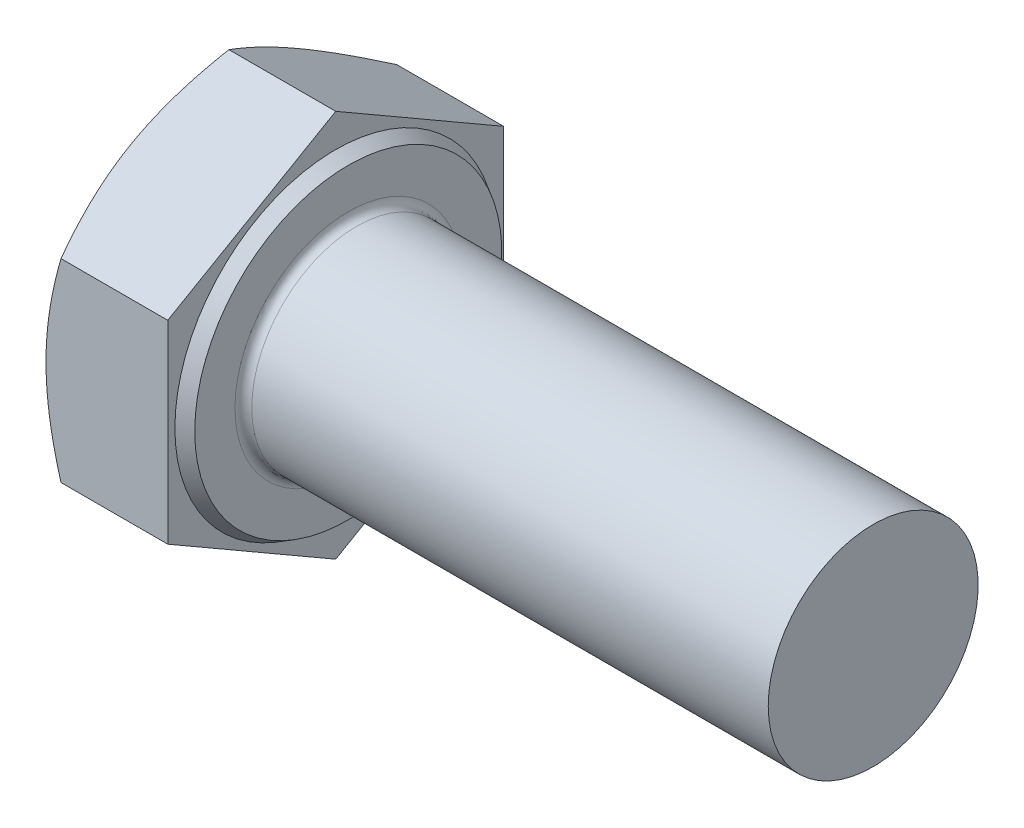
from build123d import *

# Parameters (mm, degrees)
EXTRUDE_387_DEPTH = 6.4
FILLET_1280_R     = 0.4


with BuildPart() as part:
    # 草图1 → Extrude 387 (new body)
    with BuildSketch(Plane(origin=(0, 0, 0), x_dir=(0, 0, -1), z_dir=(1, 0, 0))):
        Polygon((8, 4.618802154), (8, -4.618802154), (0, -9.237604307), (-8, -4.618802154), (-8, 4.618802154), (0, 9.237604307), align=None)
    extrude(amount=EXTRUDE_387_DEPTH)

    # 草图2 → 凸台-旋转1 (revolve)
    with BuildSketch(Plane.XY, mode=Mode.PRIVATE) as revolve_1_sk:
        Polygon((0, 0), (31.4, 0), (31.4, 3.701), (31.4, 5), (16.4, 5), (0, 5), align=None)
    revolve(revolve_1_sk.sketch.rotate(Axis((0, 0, 0), (1, 0, 0)), 90), axis=Axis((0, 0, 0), (1, 0, 0)))

    # 草图3 → 切除-旋转1 (revolve, cut)
    with BuildSketch(Plane.XY):
        Polygon((0, 8), (3.601282526, 14.237604307), (3.601282526, 19.237604307), (-10, 19.237604307), (-10, 8), align=None)
    revolve(axis=Axis((0, 0, 0), (1, 0, 0)), mode=Mode.SUBTRACT)

    # 草图4 → 切除-旋转3 (revolve, cut)
    with BuildSketch(Plane.XY, mode=Mode.PRIVATE) as cut_revolve_3_sk:
        Polygon((6.4, 7.315), (5.8, 7.661410162), (5.8, 9.237604307), (6.4, 9.237604307), align=None)
    revolve(cut_revolve_3_sk.sketch.rotate(Axis((0, 0, 0), (1, 0, 0)), 90), axis=Axis((0, 0, 0), (1, 0, 0)), mode=Mode.SUBTRACT)

    # Fillet 1280
    fillet_1280_edges = [part.edges().sort_by_distance(p)[0] for p in [
        (6.4, 0, -5),
    ]]
    fillet(fillet_1280_edges, radius=FILLET_1280_R)


solid = part.part
